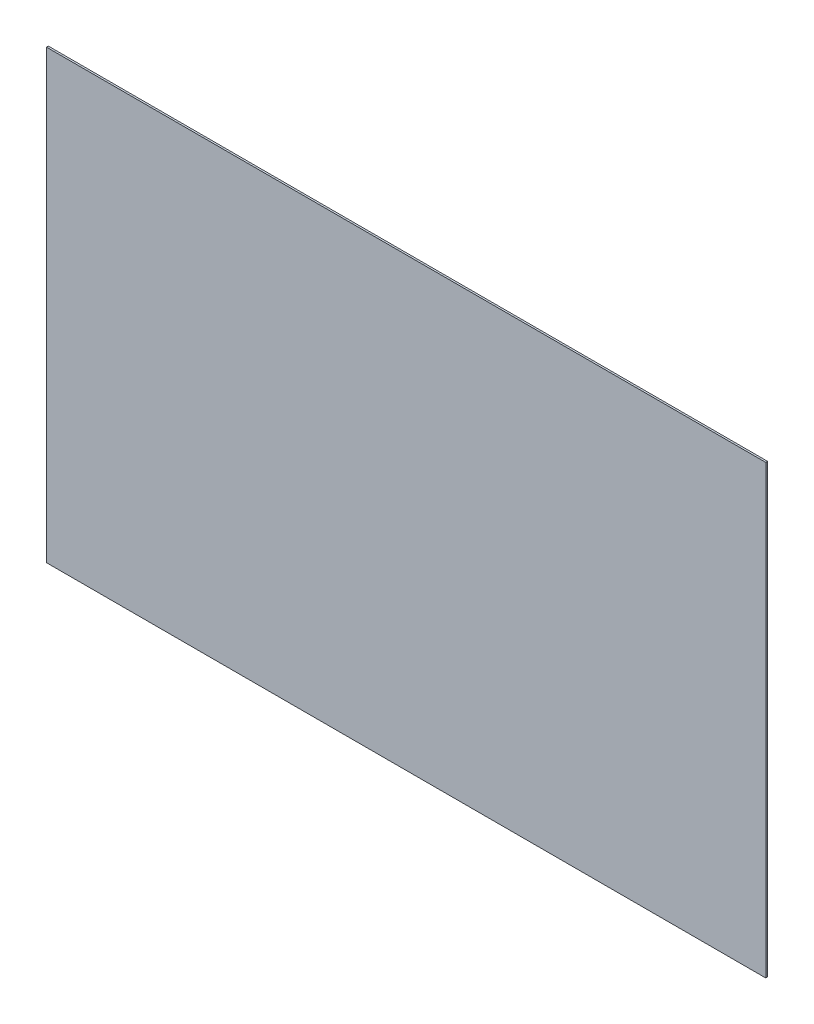
SolidWorks part; units mm, degrees
ref_plane "前视基准面" through (0, 0, 0) normal (0, 0, 1) x (1, 0, 0)
ref_plane "上视基准面" through (0, 0, 0) normal (0, 1, 0) x (1, 0, 0)
ref_plane "右视基准面" through (0, 0, 0) normal (1, 0, 0) x (0, 0, -1)
other "Configuration Table"
sketch "草图1" plane through (0, 0, 0) normal (0, 0, 1) x (1, 0, 0)
  line L1 (-580, -360) -> (580, -360)
  line L2 (-580, -360) -> (-580, 360)
  line L3 (-580, 360) -> (580, 360)
  line L4 (580, -360) -> (580, 360)
  line L5 (-580, -360) -> (580, 360) construction
  line L6 (-580, 360) -> (580, -360) construction
  point P0 (0, 0)
  dimension "D1" = 720
  dimension "D2" = 1160
extrude "凸台-拉伸1" add sketch "草图1" along normal blind 3
